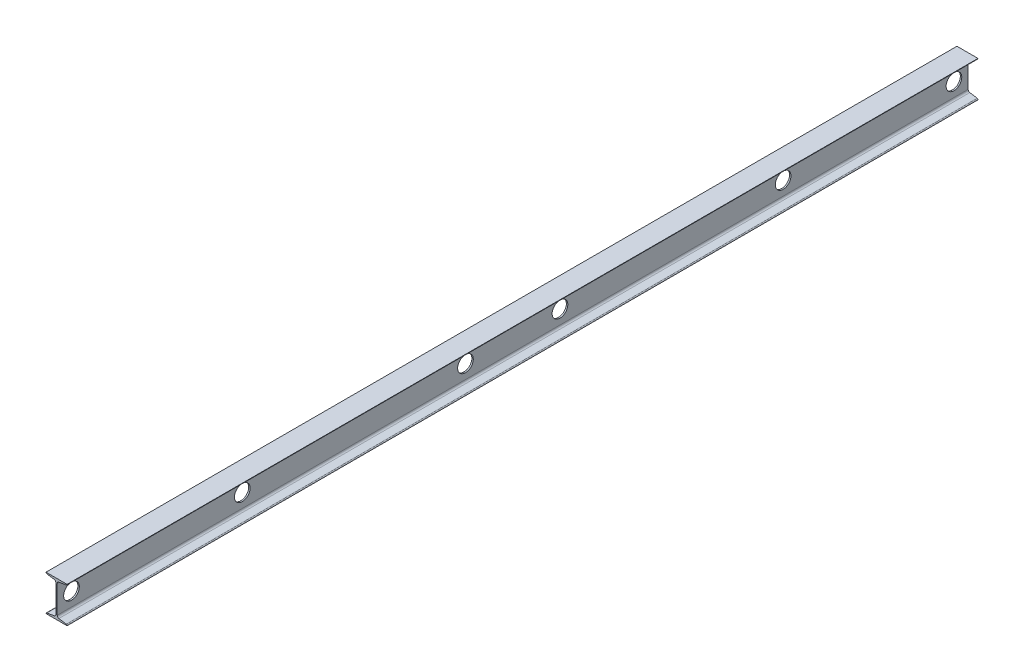
from build123d import *

# Parameters (mm, degrees)
BOSS_EXTRUDE1_DEPTH = 3200
CUT_EXTRUDE1_REACH  = 3202.864
SKETCH2_R           = 27.5


with BuildPart() as part:
    # Sketch1 → Boss-Extrude1 (new body)
    with BuildSketch(Plane.XY):
        with BuildLine():
            Line((-2.5, 48.4), (-2.5, -48.4))
            ThreePointArc((-2.5, -48.4), (-4.162700532, -52.929153828), (-8.360924112, -55.306700089))
            Line((-8.360924112, -55.306700089), (-34.069537944, -59.546649955))
            ThreePointArc((-34.069537944, -59.546649955), (-36.168649734, -60.735423086), (-37, -63))
            Line((-37, -63), (37, -63))
            ThreePointArc((37, -63), (36.168649734, -60.735423086), (34.069537944, -59.546649955))
            Line((34.069537944, -59.546649955), (8.360924112, -55.306700089))
            ThreePointArc((8.360924112, -55.306700089), (4.162700532, -52.929153828), (2.5, -48.4))
            Line((2.5, -48.4), (2.5, 48.4))
            ThreePointArc((2.5, 48.4), (4.162700532, 52.929153828), (8.360924112, 55.306700089))
            Line((8.360924112, 55.306700089), (34.069537944, 59.546649955))
            ThreePointArc((34.069537944, 59.546649955), (36.168649734, 60.735423086), (37, 63))
            Line((37, 63), (-37, 63))
            ThreePointArc((-37, 63), (-36.168649734, 60.735423086), (-34.069537944, 59.546649955))
            Line((-34.069537944, 59.546649955), (-8.360924112, 55.306700089))
            ThreePointArc((-8.360924112, 55.306700089), (-4.162700532, 52.929153828), (-2.5, 48.4))
        make_face()
    extrude(amount=BOSS_EXTRUDE1_DEPTH)

    # Sketch2 → Cut-Extrude1 (cut, up to next)
    with BuildSketch(Plane(origin=(2.5, 0, 0), x_dir=(0, 0, -1), z_dir=(1, 0, 0)), mode=Mode.PRIVATE) as cut_extrude1_sk1:
        with Locations(Location((-50, 0, 0), (0, 0, 90))):
            Circle(SKETCH2_R)
    cut_extrude1_tool1 = extrude(cut_extrude1_sk1.sketch, amount=-CUT_EXTRUDE1_REACH, mode=Mode.PRIVATE) & part.part
    # Sketch2 → Cut-Extrude1 (cut, up to next)
    with BuildSketch(Plane(origin=(2.5, 0, 0), x_dir=(0, 0, -1), z_dir=(1, 0, 0)), mode=Mode.PRIVATE) as cut_extrude1_sk2:
        with Locations(Location((-650, 0, 0), (0, 0, 90))):
            Circle(SKETCH2_R)
    cut_extrude1_tool2 = extrude(cut_extrude1_sk2.sketch, amount=-CUT_EXTRUDE1_REACH, mode=Mode.PRIVATE) & part.part
    # Sketch2 → Cut-Extrude1 (cut, up to next)
    with BuildSketch(Plane(origin=(2.5, 0, 0), x_dir=(0, 0, -1), z_dir=(1, 0, 0)), mode=Mode.PRIVATE) as cut_extrude1_sk3:
        with Locations(Location((-1434, 0, 0), (0, 0, 90))):
            Circle(SKETCH2_R)
    cut_extrude1_tool3 = extrude(cut_extrude1_sk3.sketch, amount=-CUT_EXTRUDE1_REACH, mode=Mode.PRIVATE) & part.part
    # Sketch2 → Cut-Extrude1 (cut, up to next)
    with BuildSketch(Plane(origin=(2.5, 0, 0), x_dir=(0, 0, -1), z_dir=(1, 0, 0)), mode=Mode.PRIVATE) as cut_extrude1_sk4:
        with Locations(Location((-1766, 0, 0), (0, 0, 90))):
            Circle(SKETCH2_R)
    cut_extrude1_tool4 = extrude(cut_extrude1_sk4.sketch, amount=-CUT_EXTRUDE1_REACH, mode=Mode.PRIVATE) & part.part
    # Sketch2 → Cut-Extrude1 (cut, up to next)
    with BuildSketch(Plane(origin=(2.5, 0, 0), x_dir=(0, 0, -1), z_dir=(1, 0, 0)), mode=Mode.PRIVATE) as cut_extrude1_sk5:
        with Locations(Location((-2550, 0, 0), (0, 0, 90))):
            Circle(SKETCH2_R)
    cut_extrude1_tool5 = extrude(cut_extrude1_sk5.sketch, amount=-CUT_EXTRUDE1_REACH, mode=Mode.PRIVATE) & part.part
    # Sketch2 → Cut-Extrude1 (cut, up to next)
    with BuildSketch(Plane(origin=(2.5, 0, 0), x_dir=(0, 0, -1), z_dir=(1, 0, 0)), mode=Mode.PRIVATE) as cut_extrude1_sk6:
        with Locations(Location((-3150, 0, 0), (0, 0, 90))):
            Circle(SKETCH2_R)
    cut_extrude1_tool6 = extrude(cut_extrude1_sk6.sketch, amount=-CUT_EXTRUDE1_REACH, mode=Mode.PRIVATE) & part.part
    add(cut_extrude1_tool1.solids().sort_by_distance((2.5, 0, 50))[0], mode=Mode.SUBTRACT)
    add(cut_extrude1_tool2.solids().sort_by_distance((2.5, 0, 650))[0], mode=Mode.SUBTRACT)
    add(cut_extrude1_tool3.solids().sort_by_distance((2.5, 0, 1434))[0], mode=Mode.SUBTRACT)
    add(cut_extrude1_tool4.solids().sort_by_distance((2.5, 0, 1766))[0], mode=Mode.SUBTRACT)
    add(cut_extrude1_tool5.solids().sort_by_distance((2.5, 0, 2550))[0], mode=Mode.SUBTRACT)
    add(cut_extrude1_tool6.solids().sort_by_distance((2.5, 0, 3150))[0], mode=Mode.SUBTRACT)


solid = part.part
